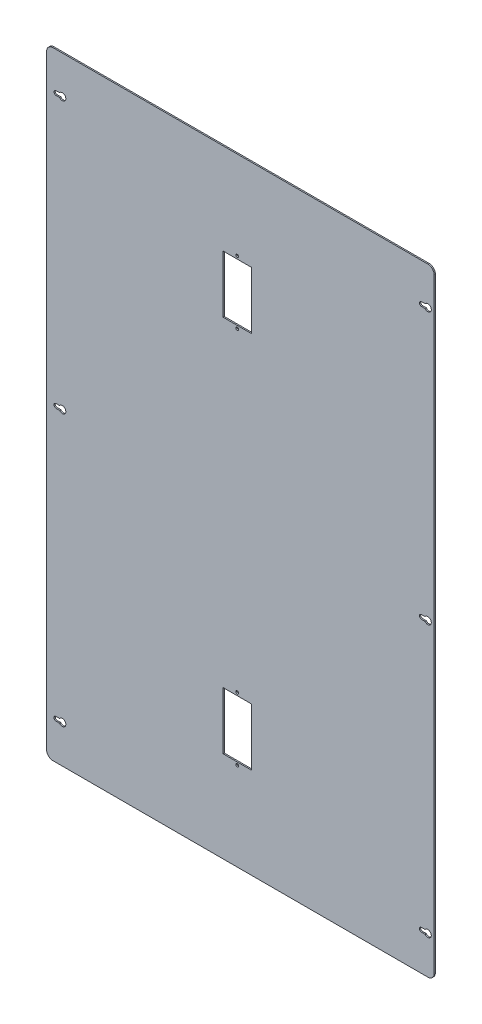
SolidWorks part; units mm, degrees
material "SPCC"
ref_plane "Front Plane" through (0, 0, 0) normal (0, 0, 1) x (1, 0, 0)
ref_plane "Top Plane" through (0, 0, 0) normal (0, 1, 0) x (1, 0, 0)
ref_plane "Right Plane" through (0, 0, 0) normal (1, 0, 0) x (0, 0, -1)
sketch "Sketch1" plane through (0, 0, 0) normal (0, 0, 1) x (1, 0, 0)
  line L1 (-307.5, 490) -> (307.5, 490)
  line L2 (-307.5, 490) -> (-307.5, -490)
  line L3 (-307.5, -490) -> (307.5, -490)
  line L4 (307.5, 490) -> (307.5, -490)
  line L5 (-307.5, 490) -> (307.5, -490) construction
  line L6 (-307.5, -490) -> (307.5, 490) construction
  point P0 (0, 0)
  dimension "D1" = 615
  dimension "D2" = 980
extrude "Boss-Extrude1" add sketch "Sketch1" along normal blind 2
sketch "Sketch7" plane through (0, 0, 0) normal (0, 0, -1) x (-1, 0, 0)
  line L1 (-17.5, 345.5) -> (27.5, 345.5)
  line L2 (-17.5, 345.5) -> (-17.5, 254.5)
  line L3 (-17.5, 254.5) -> (27.5, 254.5)
  line L4 (27.5, 345.5) -> (27.5, 254.5)
  line L5 (-17.5, 345.5) -> (27.5, 254.5) construction
  line L6 (-17.5, 254.5) -> (27.5, 345.5) construction
  line L7 (-17.5, -254.5) -> (27.5, -254.5)
  line L8 (-17.5, -254.5) -> (-17.5, -345.5)
  line L9 (-17.5, -345.5) -> (27.5, -345.5)
  line L10 (27.5, -254.5) -> (27.5, -345.5)
  line L11 (-17.5, -254.5) -> (27.5, -345.5) construction
  line L12 (-17.5, -345.5) -> (27.5, -254.5) construction
  point P0 (5, 300)
  point P5 (5, -300)
  dimension "D1" = 5
  dimension "D2" = 91
  dimension "D3" = 45
  dimension "D4" = 300
  dimension "D5" = 300
extrude "Cut-Extrude4" cut sketch "Sketch7" against normal through all
sketch "Sketch8" plane through (0, 0, 0) normal (0, 0, -1) x (-1, 0, 0)
  line L0 (5, -345.5) -> (5, -254.5) construction
  line L1 (-17.5, -345.5) -> (27.5, -345.5) construction
  line L2 (27.5, -254.5) -> (-17.5, -254.5) construction
  line L3 (-17.5, 254.5) -> (27.5, 254.5) construction
  circle A0 centre (5, 350) radius 2.25
  circle A1 centre (5, 250) radius 2.25
  circle A2 centre (5, -250) radius 2.25
  circle A3 centre (5, -350) radius 2.25
  dimension "D1" = 100
  dimension "D2" = 4.5
  dimension "D3" = 4.5
  dimension "D4" = 100
  dimension "D5" = 4.5
extrude "Cut-Extrude5" cut sketch "Sketch8" against normal through all
fillet "Fillet3" radius 10 4 edges at (307.5, -490, 1) (307.5, 490, 1) (-307.5, 490, 1) (-307.5, -490, 1)
sketch "Sketch10" plane through (0, 0, 0) normal (0, 0, -1) x (-1, 0, 0)
  line L0 (-297.5, 490) -> (297.5, 490) construction
  line L1 (307.5, 480) -> (307.5, -480) construction
  line L2 (292.5, 433.3) -> (286.9, 433.3)
  line L3 (292.5, 426.7) -> (286.9, 426.7)
  arc A0 (292.5, 426.7) -> (292.5, 433.3) centre (292.5, 430) ccw
  arc A1 (286.9, 433.3) -> (286.9, 426.7) centre (282.5, 430) ccw
  dimension "D4" = 11
  dimension "D5" = 6.6
  dimension "D1" = 60
  dimension "D2" = 15
  dimension "D3" = 10
extrude "Cut-Extrude6" cut sketch "Sketch10" against normal blind 10
pattern_linear "LPattern1" count 3 spacing 430 along (0, -1, 0) count 2 spacing 580 along (1, 0, 0) of "Cut-Extrude6"
sketch "Sketch11" plane through (0, 0, 2) normal (0, 0, 1) x (1, 0, 0)
  line L0 (-297.5, -490) -> (297.5, -490) construction
  line L1 (97.5, 520) -> (247.5, 520)
  line L2 (97.5, 520) -> (97.5, 270)
  line L3 (97.5, 270) -> (247.5, 270)
  line L4 (247.5, 520) -> (247.5, 270)
  line L5 (97.5, -180) -> (247.5, -180)
  line L6 (97.5, -180) -> (97.5, -410)
  line L7 (97.5, -410) -> (247.5, -410)
  line L8 (247.5, -180) -> (247.5, -410)
  line L9 (307.5, -480) -> (307.5, 480) construction
  dimension "D1" = 80
  dimension "D2" = 230
  dimension "D3" = 450
  dimension "D4" = 250
  dimension "D5" = 60
  dimension "D6" = 150
extrude "Cut-Extrude7" [suppressed] cut sketch "Sketch11" against normal through all
